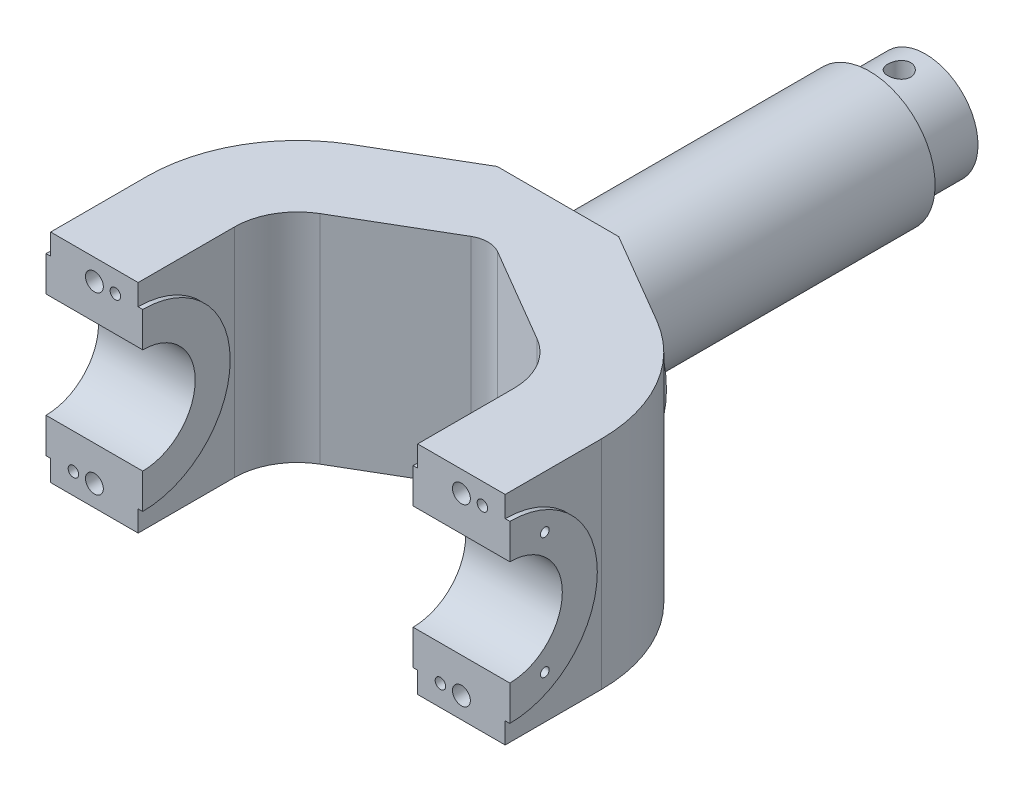
SolidWorks part; units mm, degrees
material "35"
ref_plane "Front Plane" through (0, 0, 0) normal (0, 0, 1) x (1, 0, 0)
ref_plane "Top Plane" through (0, 0, 0) normal (0, 1, 0) x (1, 0, 0)
ref_plane "Right Plane" through (0, 0, 0) normal (1, 0, 0) x (0, 0, -1)
sketch "Sketch1" plane through (0, 0, 0) normal (0, 1, 0) x (1, 0, 0)
  line L0 (-367.6336, 0) -> (466.5649, 0) construction
  line L1 (0, 287.0229) -> (0, -151.4504) construction
  line L2 (-374.9618, -160) -> (459.2366, -160) construction
  line L3 (-129.85, -160) -> (-79.85, -160)
  line L4 (-79.85, -160) -> (-79.85, -105)
  line L5 (-129.85, -160) -> (-129.85, -105)
  line L6 (-87.2938, -30.7798) -> (-34.709, 0)
  line L7 (-62.0358, -73.9311) -> (-7.5774, -42.0546)
  line L8 (62.0358, -73.9311) -> (7.5774, -42.0546)
  line L9 (87.2938, -30.7798) -> (34.709, 0)
  line L10 (129.85, -160) -> (129.85, -105)
  line L11 (79.85, -160) -> (79.85, -105)
  line L12 (129.85, -160) -> (79.85, -160)
  line L13 (-34.709, 0) -> (34.709, 0)
  arc A0 (79.85, -105) -> (62.0358, -73.9311) centre (43.85, -105) ccw
  arc A1 (-79.85, -105) -> (-62.0358, -73.9311) centre (-43.85, -105) cw
  arc A2 (129.85, -105) -> (87.2938, -30.7798) centre (43.85, -105) ccw
  arc A3 (-129.85, -105) -> (-87.2938, -30.7798) centre (-43.85, -105) cw
  arc A4 (7.5774, -42.0546) -> (-7.5774, -42.0546) centre (0, -55) ccw
  point P21 (79.85, -84.3584)
  point P24 (-79.85, -84.3584)
  point P27 (129.85, -55.6895)
  point P30 (-129.85, -55.6895)
  dimension "D2" = 55
  dimension "D3" = 36
  dimension "D4" = 15
  dimension "D8" = 86
  dimension "D1" = 160
  dimension "D5" = 105
  dimension "D6" = 159.7
  dimension "D7" = 50
  dimension "D9" = 50
extrude "Boss-Extrude1" add sketch "Sketch1" along normal mid plane 124
sketch "Sketch2" plane through (0, 0, 0) normal (0, 0, 1) x (1, 0, 0)
  circle A0 centre (0, 0) radius 62
  dimension "D1" = 124
extrude "Boss-Extrude2" add sketch "Sketch2" along normal up to next
sketch "Sketch3" plane through (0, 0, 0) normal (0, 0, 1) x (1, 0, 0)
  circle A0 centre (0, 0) radius 37.5
  dimension "D1" = 75
extrude "Boss-Extrude3" add sketch "Sketch3" against normal blind 178
sketch "Sketch4" plane through (0, 0, 0) normal (0, 0, 1) x (1, 0, 0)
  circle A0 centre (0, 0) radius 30
  dimension "D1" = 60
extrude "Boss-Extrude4" add sketch "Sketch4" against normal blind 210
sketch "Sketch5" plane through (0, 0, 0) normal (0, 1, 0) x (1, 0, 0)
  line L0 (0, 84.1381) -> (0, -36.1542) construction
  circle A0 centre (0, 195) radius 6.5
  dimension "D2" = 13
  dimension "D1" = 195
extrude "Cut-Extrude1" cut sketch "Sketch5" against normal through all both and the other way through all
sketch "Sketch6" plane through (0, 0, 0) normal (1, 0, 0) x (0, 0, -1)
  line L0 (-160, 62) -> (-160, -62) construction
  line L1 (-160, 50) -> (-160, 30)
  line L2 (-182.0463, 0) -> (42.1672, 0) construction
  line L3 (-160, -30) -> (-160, -50)
  arc A0 (-160, 30) -> (-160, -30) centre (-160, 0) cw
  arc A1 (-160, 50) -> (-160, -50) centre (-160, 0) cw
  dimension "D1" = 30
  dimension "D2" = 50
extrude "Boss-Extrude5" add sketch "Sketch6" along normal mid plane 265
sketch "Sketch7" plane through (0, 0, 0) normal (1, 0, 0) x (0, 0, -1)
  line L0 (-160, 28) -> (-160, 52)
  line L1 (-160, -28) -> (-160, -52)
  arc A0 (-160, -50) -> (-160, 50) centre (-160, 0) ccw construction
  arc A1 (-160, -30) -> (-160, 30) centre (-160, 0) ccw construction
  arc A2 (-160, -50) -> (-160, 50) centre (-160, 0) ccw construction
  arc A3 (-160, -30) -> (-160, 30) centre (-160, 0) ccw construction
  arc A4 (-160, -28) -> (-160, 28) centre (-160, 0) ccw
  arc A5 (-160, -52) -> (-160, 52) centre (-160, 0) ccw
  dimension "D1" = 2
  dimension "D2" = 2
extrude "Cut-Extrude2" cut sketch "Sketch7" against normal mid plane 154.5
sketch "Sketch15" plane through (0, 0, 0) normal (1, 0, 0) x (0, 0, -1)
  line L0 (-160, 30) -> (-160, -30) construction
  line L1 (-160, 30) -> (-160, -30)
  arc A0 (-160, -30) -> (-160, 30) centre (-160, 0) ccw construction
  arc A1 (-160, -30) -> (-160, 30) centre (-160, 0) ccw
extrude "Cut-Extrude3" cut sketch "Sketch15" against normal through all both and the other way through all
hole_wizard "M6 Tapped Hole1" positions "Sketch9" profile "Sketch8" tap size "M6" standard "GB"
sketch "Sketch9" plane through (132.5, 0, 0) normal (1, 0, 0) x (0, 0, -1)
  line L0 (-170.541, -18.2575) -> (-103.5459, 97.7814) construction
  line L2 (-230.1687, 0) -> (261.7715, 0) construction
  line L4 (-170.541, 18.2575) -> (-103.5459, -97.7814) construction
  arc A0 (-160, -30) -> (-160, 30) centre (-160, 0) ccw construction
  arc A1 (-160, -30) -> (-160, 30) centre (-160, 0) ccw construction
  arc A2 (-160, -40) -> (-160, 40) centre (-160, 0) ccw construction
  point P0 (-140, 34.641)
  point P2 (-140, -34.641)
  dimension "D1" = 40
  dimension "D2" = 60
sketch "Sketch8" plane through (132.5, 34.641, 140) normal (0, 1, 0) x (0, 0, -1)
  line L0 (0, 0) -> (0, 18.5022)
  line L1 (0, 18.5022) -> (2.5, 17)
  line L2 (2.5, 17) -> (2.5, 0)
  line L5 (2.5, 0) -> (0, 0)
  line L10 (0, 18.5022) -> (-2.5, 17) construction
  line L11 (0, -6.35) -> (0, 107.95) construction
  dimension "螺纹孔钻头直径" = 5
  dimension "螺纹孔钻头深度" = 17
  dimension "导头角度" = 118
cosmetic thread "Cosmetic Thread9" parameters "D1"=12, "D2"=6
cosmetic thread "Cosmetic Thread10" parameters "D1"=12, "D2"=6
mirror "Mirror1" about plane through (0, 0, 0) normal (1, 0, 0) of "M6 Tapped Hole1"
hole_wizard "M12 Tapped Hole1" positions "Sketch11" profile "Sketch10" tap size "M12" standard "GB"
sketch "Sketch11" plane through (0, 0, 160) normal (0, 0, 1) x (1, 0, 0)
  line L0 (79.85, 62) -> (129.85, 62) construction
  line L1 (79.85, -62) -> (129.85, -62) construction
  line L2 (79.85, 62) -> (129.85, 62) construction
  line L3 (79.85, -62) -> (129.85, -62) construction
  line L4 (104.85, 62) -> (104.85, -62) construction
  line L6 (-154.0751, 0) -> (162.8962, 0) construction
  line L7 (-104.85, 62) -> (-104.85, -62) construction
  line L8 (-129.85, 62) -> (-79.85, 62) construction
  line L9 (-129.85, -62) -> (-79.85, -62) construction
  point P0 (104.85, 50)
  point P2 (104.85, -50)
  point P25 (-104.85, 50)
  point P27 (-104.85, -50)
  dimension "D1" = 100
  dimension "D2" = 100
sketch "Sketch10" plane through (104.85, 50, 160) normal (1, 0, 0) x (0, -1, 0)
  line L0 (0, 0) -> (0, 39.8144)
  line L1 (0, 39.8144) -> (5.1, 36.75)
  line L2 (5.1, 36.75) -> (5.1, 0)
  line L5 (5.1, 0) -> (0, 0)
  line L10 (0, 39.8144) -> (-5.1, 36.75) construction
  line L11 (0, -6.35) -> (0, 107.95) construction
  dimension "螺纹孔钻头直径" = 10.2
  dimension "螺纹孔钻头深度" = 36.75
  dimension "导头角度" = 118
cosmetic thread "Cosmetic Thread3" parameters "D1"=28, "D2"=12
cosmetic thread "Cosmetic Thread4" parameters "D1"=28, "D2"=12
cosmetic thread "Cosmetic Thread5" parameters "D1"=28, "D2"=12
cosmetic thread "Cosmetic Thread6" parameters "D1"=28, "D2"=12
hole_wizard "6mm blind pin hole1" positions "Sketch14" profile "Sketch13" hole size "Ø6.0" standard "GB"
sketch "Sketch14" plane through (0, 0, 160) normal (0, 0, 1) x (1, 0, 0)
  line L0 (79.85, 62) -> (129.85, 62) construction
  line L1 (79.85, -62) -> (129.85, -62) construction
  line L2 (79.85, 62) -> (129.85, 62) construction
  line L3 (79.85, -62) -> (129.85, -62) construction
  line L4 (104.85, 62) -> (104.85, -62) construction
  line L6 (-189.6962, 0) -> (172.4335, 0) construction
  line L7 (-104.85, 62) -> (-104.85, -62) construction
  line L8 (-129.85, 62) -> (-79.85, 62) construction
  line L9 (-129.85, -62) -> (-79.85, -62) construction
  point P0 (116.85, 50)
  point P2 (92.85, -50)
  point P21 (-92.85, 50)
  point P23 (-116.85, -50)
  dimension "D1" = 12
  dimension "D2" = 12
  dimension "D3" = 100
  dimension "D4" = 50
  dimension "D5" = 12
  dimension "D6" = 12
  dimension "D7" = 100
  dimension "D8" = 50
sketch "Sketch13" plane through (116.85, 50, 160) normal (1, 0, 0) x (0, -1, 0)
  line L0 (0, 0) -> (0, 16.8026)
  line L1 (0, 16.8026) -> (3, 15)
  line L2 (3, 15) -> (3, 0)
  line L5 (3, 0) -> (0, 0)
  line L10 (0, 16.8026) -> (-3, 15) construction
  line L11 (0, -6.35) -> (0, 107.95) construction
  dimension "孔直径" = 6
  dimension "孔深度" = 15
  dimension "导头角度" = 118
chamfer "Chamfer1" distance 2 angle 45 1 edges at (30, 0, -178)
fillet "Fillet1" radius 3 1 edges at (37.5, 0, 0)
